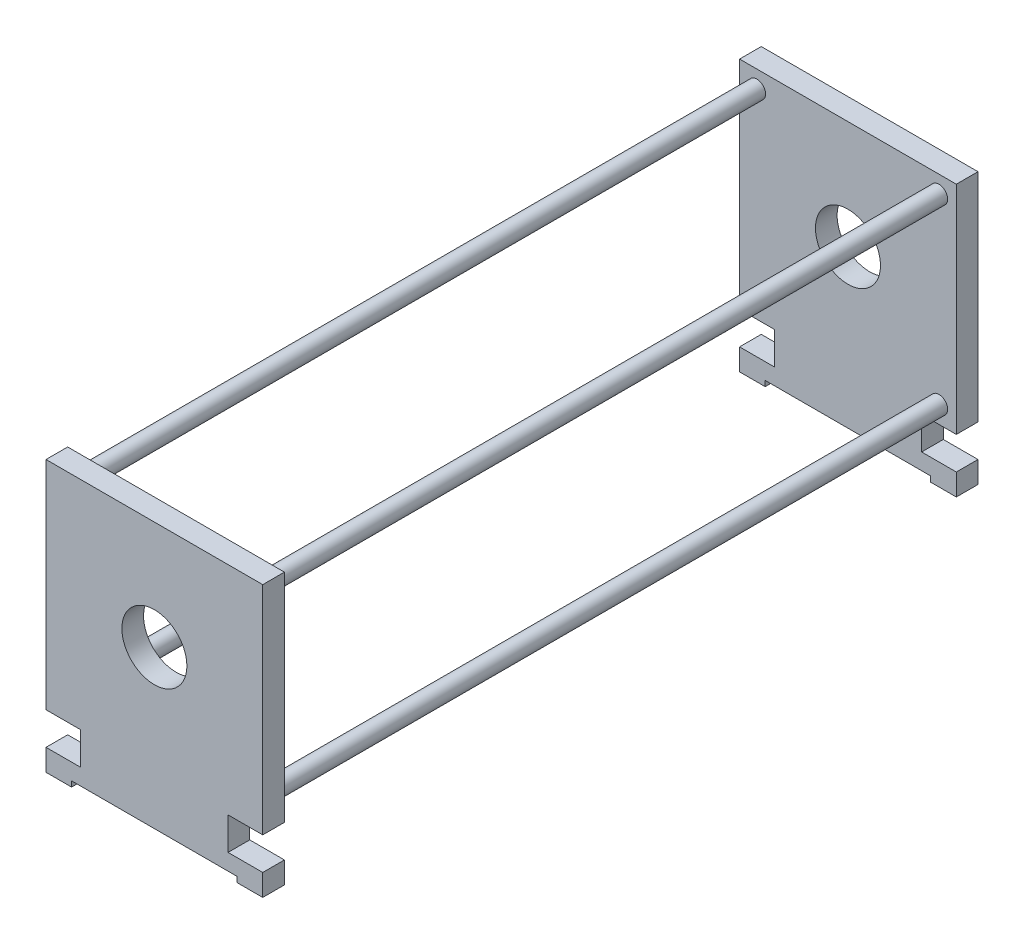
SolidWorks part; units mm, degrees
ref_plane "Front Plane" through (0, 0, 0) normal (0, 0, 1) x (1, 0, 0)
ref_plane "Top Plane" through (0, 0, 0) normal (0, 1, 0) x (1, 0, 0)
ref_plane "Right Plane" through (0, 0, 0) normal (1, 0, 0) x (0, 0, -1)
sketch "Sketch1" plane through (0, 0, 0) normal (0, 0, 1) x (1, 0, 0)
  line L0 (76.3889, 0) -> (-76.3889, 0)
  line L1 (-76.3889, 0) -> (-76.3889, -5)
  line L2 (-76.3889, -5) -> (-100, -5)
  line L3 (-100, -5) -> (-100, 15)
  line L4 (-100, 15) -> (-68, 15)
  line L5 (-68, 15) -> (-68, 45)
  line L6 (-68, 45) -> (-100, 45)
  line L7 (-100, 45) -> (-100, 245)
  line L8 (-100, 245) -> (100, 245)
  line L9 (0, 0) -> (0, 160.4328) construction
  line L10 (100, 45) -> (100, 245)
  line L11 (68, 45) -> (100, 45)
  line L12 (68, 15) -> (68, 45)
  line L13 (100, 15) -> (68, 15)
  line L14 (100, -5) -> (100, 15)
  line L15 (76.3889, -5) -> (100, -5)
  line L16 (76.3889, 0) -> (76.3889, -5)
  circle A0 centre (0, 145) radius 30
  point P13 (0, 245)
  dimension "D8" = 60
  dimension "D9" = 100
  dimension "D1" = 100
  dimension "D2" = 200
  dimension "D3" = 30
  dimension "D4" = 5
  dimension "D5" = 20
  dimension "D6" = 32
  dimension "D7" = 100
extrude "Boss-Extrude1" add sketch "Sketch1" along normal blind 20
sketch "Sketch2" plane through (0, 0, 20) normal (0, 0, 1) x (1, 0, 0)
  line L0 (100, 45) -> (100, 245) construction
  line L1 (100, 245) -> (-100, 245) construction
  line L2 (-100, 245) -> (-100, 45) construction
  line L3 (-100, 45) -> (-68, 45) construction
  line L4 (68, 45) -> (100, 45) construction
  circle A0 centre (-84, 229) radius 8
  circle A1 centre (84, 229) radius 8
  circle A2 centre (84, 61) radius 8
  circle A3 centre (-84, 61) radius 8
  dimension "D1" = 16
  dimension "D2" = 16
  dimension "D3" = 16
  dimension "D4" = 16
  dimension "D5" = 16
  dimension "D6" = 16
  dimension "D7" = 16
  dimension "D8" = 16
  dimension "D9" = 16
extrude "Boss-Extrude2" add sketch "Sketch2" along normal blind 620
sketch "Sketch3" plane through (0, 0, 640) normal (0, 0, 1) x (1, 0, 0)
  line L0 (76.3889, 0) -> (-76.3889, 0)
  line L1 (-76.3889, 0) -> (-76.3889, -5)
  line L2 (-76.3889, -5) -> (-100, -5)
  line L3 (-100, -5) -> (-100, 15)
  line L4 (-100, 15) -> (-68, 15)
  line L5 (-68, 15) -> (-68, 45)
  line L6 (-68, 45) -> (-100, 45)
  line L7 (-100, 45) -> (-100, 245)
  line L8 (-100, 245) -> (100, 245)
  line L9 (0, 0) -> (0, 160.4328) construction
  line L10 (100, 45) -> (100, 245)
  line L11 (68, 45) -> (100, 45)
  line L12 (68, 15) -> (68, 45)
  line L13 (100, 15) -> (68, 15)
  line L14 (100, -5) -> (100, 15)
  line L15 (76.3889, -5) -> (100, -5)
  line L16 (76.3889, 0) -> (76.3889, -5)
  line L17 (-100, 245) -> (-100, 45) construction
  line L18 (100, 245) -> (-100, 245) construction
  circle A0 centre (0, 145) radius 30
  point P12 (0, 245)
  dimension "D8" = 60
  dimension "D1" = 100
  dimension "D2" = 200
  dimension "D3" = 30
  dimension "D4" = 5
  dimension "D5" = 20
  dimension "D6" = 32
  dimension "D7" = 100
  dimension "D9" = 100
extrude "Boss-Extrude3" add sketch "Sketch3" along normal blind 20
